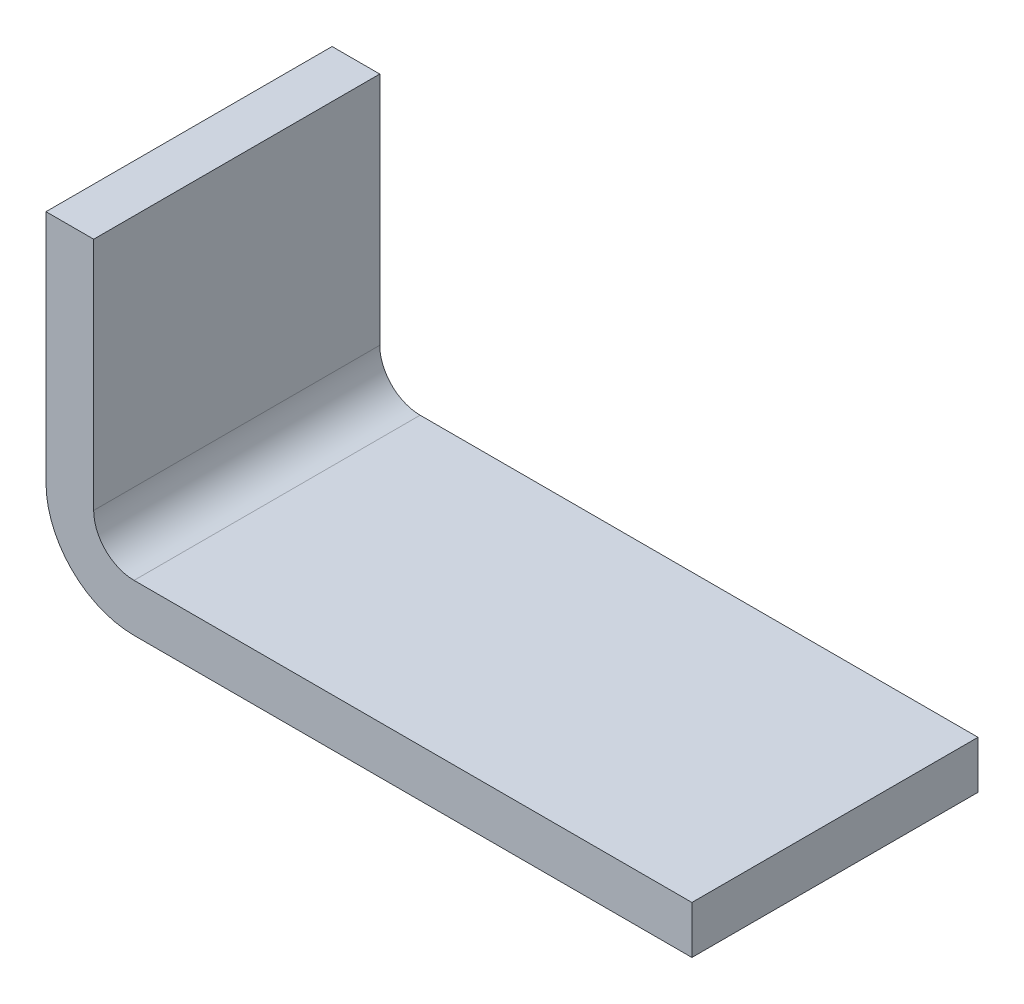
from build123d import *

# Parameters (mm, degrees)
EXTRUDE1_DEPTH = 45


with BuildPart() as part:
    # Sketch1 → Extrude1 (new body)
    with BuildSketch(Plane.XY):
        with BuildLine():
            Line((-23.952923538, 5.356071964), (-23.952923538, -31.593928036))
            ThreePointArc((-23.952923538, -31.593928036), (-19.896352458, -41.387356955), (-10.102923538, -45.443928036))
            Line((-10.102923538, -45.443928036), (77.647076462, -45.443928036))
            Line((77.647076462, -45.443928036), (77.647076462, -37.943928036))
            Line((77.647076462, -37.943928036), (-10.102923538, -37.943928036))
            ThreePointArc((-10.102923538, -37.943928036), (-14.593051599, -36.084056097), (-16.452923538, -31.593928036))
            Line((-16.452923538, -31.593928036), (-16.452923538, 5.356071964))
            Line((-16.452923538, 5.356071964), (-23.952923538, 5.356071964))
        make_face()
    extrude(amount=EXTRUDE1_DEPTH)


solid = part.part
